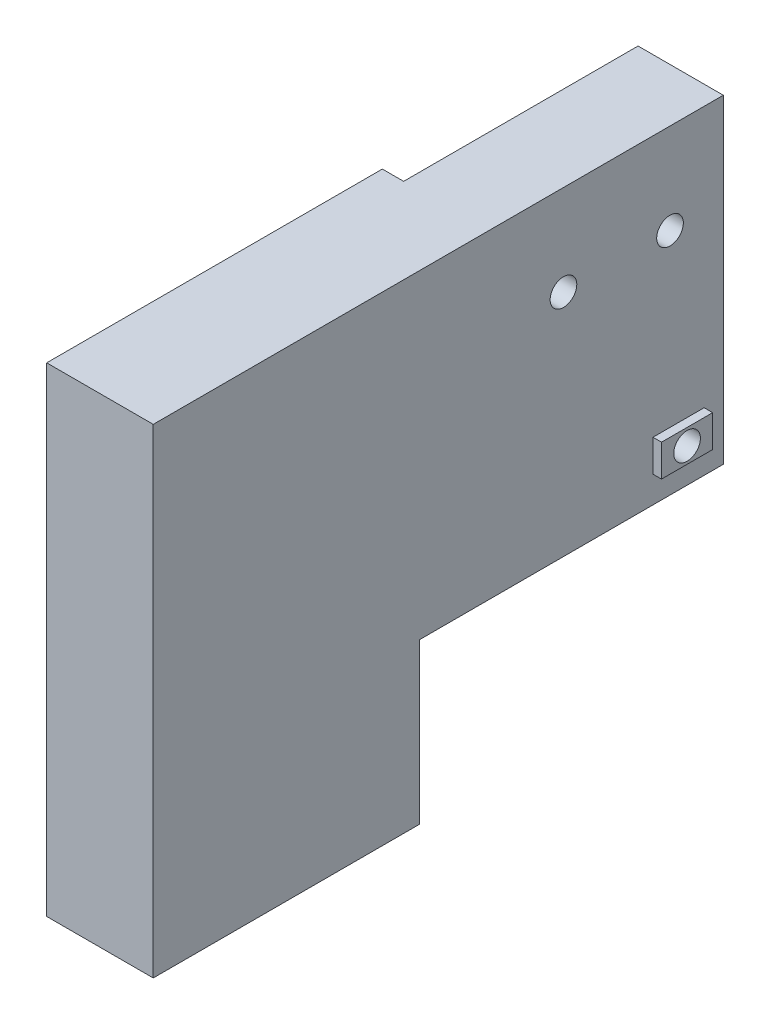
from build123d import *

# Parameters (mm, degrees)
EXTRUDE_THIN1_DEPTH   = 25
SKETCH2_W             = 28.5
SKETCH2_H             = 30
BOSS_EXTRUDE1_DEPTH   = 10
SKETCH5_W             = 2
SKETCH5_H             = 22
CUT_EXTRUDE1_DEPTH    = 64.735782728
M3_TAPPED_HOLE2_D     = 2.5
SKETCH8_W             = 85.55195354
SKETCH8_H             = 65.589831047
CUT_EXTRUDE2_DEPTH    = 10
M5_TAPPED_HOLE1_D     = 4.2
M5_TAPPED_HOLE1_DEPTH = 12.4
M5_TAPPED_HOLE1_TIP   = 1.2618073
SKETCH14_W            = 4.8
SKETCH14_H            = 3
BOSS_EXTRUDE2_DEPTH   = 0.8
M3_TAPPED_HOLE1_D     = 2.5


with BuildPart() as part:
    # Sketch1 → Extrude-Thin1 (new body)
    with BuildSketch(Plane.XY):
        Polygon((-15, 0), (0, 0), (0, 45), (10, 45), (10, -10), (-15, -10), align=None)
    extrude(amount=EXTRUDE_THIN1_DEPTH)

    # Sketch2 → Boss-Extrude1 (add)
    with BuildSketch(Plane.ZY):
        with Locations((-14.25, 30)):
            Rectangle(SKETCH2_W, SKETCH2_H)
    extrude(amount=-BOSS_EXTRUDE1_DEPTH)

    # Sketch5 → Cut-Extrude1 (cut, through all)
    with BuildSketch(Plane(origin=(0, 45, 0), x_dir=(1, 0, 0), z_dir=(0, 1, 0))):
        with Locations((1, 17.5)):
            Rectangle(SKETCH5_W, SKETCH5_H)
    extrude(amount=-CUT_EXTRUDE1_DEPTH, mode=Mode.SUBTRACT)

    # M3 Tapped Hole2 (through all)
    with Locations(Plane(origin=(10, 0, 0), x_dir=(0, 0, -1), z_dir=(1, 0, 0))):
        with Locations((13.5, 36.5), (23.5, 36.5)):
            Hole(M3_TAPPED_HOLE2_D / 2)

    # Sketch8 → Cut-Extrude2 (cut)
    with BuildSketch(Plane.XZ.offset(10)):
        with Locations((-7.814591053, 5.120081117)):
            Rectangle(SKETCH8_W, SKETCH8_H)
    extrude(amount=-CUT_EXTRUDE2_DEPTH, mode=Mode.SUBTRACT)

    # M5 Tapped Hole1
    with Locations(Plane(origin=(0, 0, 0), x_dir=(-1, 0, 0), z_dir=(0, -1, 0))):
        with Locations((-5, -5.5), (-5, -19.5)):
            Hole(M5_TAPPED_HOLE1_D / 2, depth=M5_TAPPED_HOLE1_DEPTH)
            with Locations((0, 0, -(M5_TAPPED_HOLE1_DEPTH + M5_TAPPED_HOLE1_TIP / 2))):  # 118° drill point
                Cone(0, M5_TAPPED_HOLE1_D / 2, M5_TAPPED_HOLE1_TIP, mode=Mode.SUBTRACT)

    # Sketch14 → Boss-Extrude2 (add)
    with BuildSketch(Plane(origin=(10, 0, 0), x_dir=(0, 0, -1), z_dir=(1, 0, 0))):
        with Locations((24.3, 19)):
            Rectangle(SKETCH14_W, SKETCH14_H)
    extrude(amount=BOSS_EXTRUDE2_DEPTH)

    # M3 Tapped Hole1 (through all)
    with Locations(Plane.ZY):
        with Locations((-24.3, 19)):
            Hole(M3_TAPPED_HOLE1_D / 2)


solid = part.part
